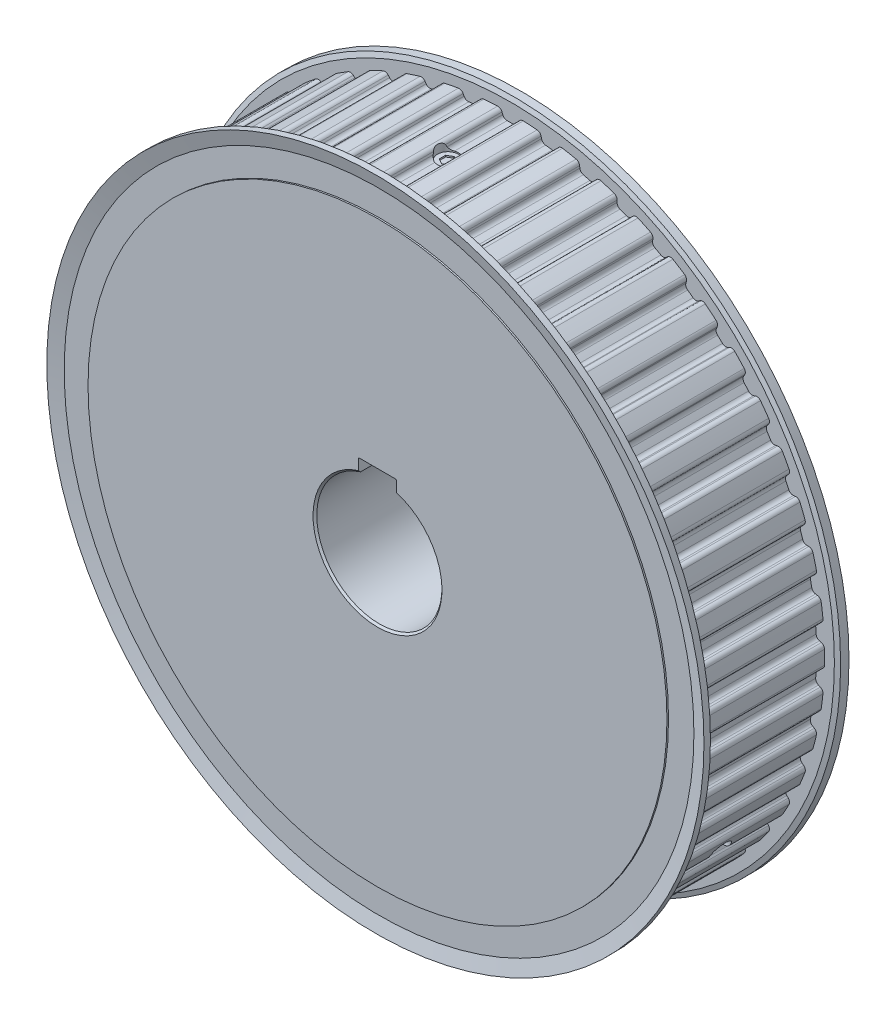
from build123d import *

# Parameters (mm, degrees)
CUT_EXTRUDE_1_DEPTH      = 20
CUT_EXTRUDE_1_DEPTH_BACK = 20
SKETCH_4_R               = 200.76
CUT_EXTRUDE_2_DEPTH      = 22.5
CUT_EXTRUDE_2_DEPTH_BACK = 22.5
SKETCH_8_W               = 3.3235
SKETCH_8_H               = 81.38
CUT_EXTRUDE_3_DEPTH      = 0.5
CUT_EXTRUDE_4_DEPTH      = 0.5


with BuildPart() as part:
    # 草图1 → 旋转1 (revolve)
    with BuildSketch(Plane(origin=(0, 0, 0), x_dir=(0, 0, -1), z_dir=(1, 0, 0)), mode=Mode.PRIVATE) as revolve_1_sk:
        Polygon((0, 0), (0, 92.5), (2.5, 92.5), (2.5, 102.38), (42.5, 102.38), (42.5, 92.5), (45, 92.5), (45, 0), align=None)
    revolve(revolve_1_sk.sketch.rotate(Axis((0, 0, -45), (0, 0, 1)), 270), axis=Axis((0, 0, -45), (0, 0, 1)))

    # 草图2 → 切除-旋转1 (revolve, cut)
    with BuildSketch(Plane(origin=(0, 0, 0), x_dir=(0, 0, -1), z_dir=(1, 0, 0)), mode=Mode.PRIVATE) as cut_revolve_1_sk:
        Polygon((0, 0), (0, 20.6), (0.6, 20), (44.4, 20), (45, 20.6), (45, 0), align=None)
    revolve(cut_revolve_1_sk.sketch.rotate(Axis((0, 0, -45), (0, 0, 1)), 270), axis=Axis((0, 0, -45), (0, 0, 1)), mode=Mode.SUBTRACT)

    # 草图3 → 旋转2 (revolve)
    with BuildSketch(Plane(origin=(0, 0, 0), x_dir=(0, 0, -1), z_dir=(1, 0, 0)), mode=Mode.PRIVATE) as revolve_2_sk:
        Polygon((42.5, 103.5), (42.5, 92.5), (44.5, 92.5), (44.5, 105), (43, 105), align=None)
    revolve(revolve_2_sk.sketch.rotate(Axis((0, 0, -50), (0, 0, 1)), 270), axis=Axis((0, 0, -50), (0, 0, 1)))

    # 草图4 → 切除-拉伸1 (cut, two sides: drawn at the far end of the back side and taken through both)
    with BuildSketch(Plane.XY.offset(-22.5).offset(-CUT_EXTRUDE_1_DEPTH_BACK)):
        Circle(SKETCH_4_R)
        with BuildLine():
            Line((-99.336884651, -3.543386548), (-98.711914642, -3.727325224))
            ThreePointArc((-98.711914642, -3.727325224), (-97.97307181, -4.226775349), (-97.658926902, -5.061432245))
            ThreePointArc((-97.658926902, -5.061432245), (-97.597033773, -6.140284905), (-97.523222764, -7.218387755))
            ThreePointArc((-97.523222764, -7.218387755), (-97.730280298, -8.085835929), (-98.400699434, -8.673949302))
            Line((-98.400699434, -8.673949302), (-98.997687739, -8.934767079))
            ThreePointArc((-98.997687739, -8.934767079), (-99.656069764, -9.521039759), (-99.841575427, -10.382880925))
            ThreePointArc((-99.841575427, -10.382880925), (-99.588473718, -12.580949985), (-99.286986225, -14.772906499))
            ThreePointArc((-99.286986225, -14.772906499), (-98.892977381, -15.561537958), (-98.109479551, -15.965658852))
            Line((-98.109479551, -15.965658852), (-97.466383988, -16.069817605))
            ThreePointArc((-97.466383988, -16.069817605), (-96.670769454, -16.472727855), (-96.254491424, -17.261430435))
            ThreePointArc((-96.254491424, -17.261430435), (-96.057870249, -18.324018753), (-95.849519145, -19.384369468))
            ThreePointArc((-95.849519145, -19.384369468), (-95.946223884, -20.270928745), (-96.537646414, -20.938430466))
            Line((-96.537646414, -20.938430466), (-97.097238152, -21.272014092))
            ThreePointArc((-97.097238152, -21.272014092), (-97.676949188, -21.936180984), (-97.752974743, -22.8144763))
            ThreePointArc((-97.752974743, -22.8144763), (-97.226377714, -24.963490874), (-96.652542542, -27.100376754))
            ThreePointArc((-96.652542542, -27.100376754), (-96.162798845, -27.833407215), (-95.334829351, -28.136143178))
            Line((-95.334829351, -28.136143178), (-94.683750235, -28.158879362))
            ThreePointArc((-94.683750235, -28.158879362), (-93.843911315, -28.458895602), (-93.332065117, -29.189205555))
            ThreePointArc((-93.332065117, -29.189205555), (-93.003816729, -30.21877188), (-92.664211352, -31.244648095))
            ThreePointArc((-92.664211352, -31.244648095), (-92.649038204, -32.136336905), (-93.152137042, -32.872700074))
            Line((-93.152137042, -32.872700074), (-93.665507117, -33.273788735))
            ThreePointArc((-93.665507117, -33.273788735), (-94.157404774, -34.005375532), (-94.122751253, -34.886273755))
            ThreePointArc((-94.122751253, -34.886273755), (-93.330963653, -36.952342598), (-92.493830526, -39.000457877))
            ThreePointArc((-92.493830526, -39.000457877), (-91.916075526, -39.666327014), (-91.056691942, -39.86290372))
            Line((-91.056691942, -39.86290372), (-90.40789718, -39.803858771))
            ThreePointArc((-90.40789718, -39.803858771), (-89.537078635, -39.996249566), (-88.937736389, -40.656649468))
            ThreePointArc((-88.937736389, -40.656649468), (-88.483037461, -41.636956922), (-88.01753359, -42.612179957))
            ThreePointArc((-88.01753359, -42.612179957), (-87.890721846, -43.494935834), (-88.297562822, -44.288547564))
            Line((-88.297562822, -44.288547564), (-88.756615082, -44.750815853))
            ThreePointArc((-88.756615082, -44.750815853), (-89.15294184, -45.538284993), (-89.00815575, -46.407893833))
            ThreePointArc((-89.00815575, -46.407893833), (-87.963664543, -48.358433806), (-86.876435549, -50.285478483))
            ThreePointArc((-86.876435549, -50.285478483), (-86.219780788, -50.87368514), (-85.342536106, -50.961002456))
            Line((-85.342536106, -50.961002456), (-84.706257579, -50.821107549))
            ThreePointArc((-84.706257579, -50.821107549), (-83.818192738, -50.902838781), (-83.14080643, -51.48291373))
            ThreePointArc((-83.14080643, -51.48291373), (-82.566827835, -52.398502281), (-81.982766745, -53.307692286))
            ThreePointArc((-81.982766745, -53.307692286), (-81.7463163, -54.167593643), (-82.05048329, -55.005938202))
            Line((-82.05048329, -55.005938202), (-82.447978207, -55.522095872))
            ThreePointArc((-82.447978207, -55.522095872), (-82.742483756, -56.353028497), (-82.489848459, -57.197633703))
            ThreePointArc((-82.489848459, -57.197633703), (-81.209125895, -59.001883625), (-79.888947287, -60.777467053))
            ThreePointArc((-79.888947287, -60.777467053), (-79.163748602, -61.27873486), (-78.282477495, -61.255415741))
            Line((-78.282477495, -61.255415741), (-77.668749695, -61.036877102))
            ThreePointArc((-77.668749695, -61.036877102), (-76.777443871, -61.00665982), (-76.032696287, -61.49726169))
            ThreePointArc((-76.032696287, -61.49726169), (-75.348490011, -62.333691958), (-74.655082694, -63.162510463))
            ThreePointArc((-74.655082694, -63.162510463), (-74.312722514, -63.985996142), (-74.509418622, -64.855852336))
            Line((-74.509418622, -64.855852336), (-74.839087463, -65.417759272))
            ThreePointArc((-74.839087463, -65.417759272), (-75.027127275, -66.279051078), (-74.670626981, -67.08533272))
            ThreePointArc((-74.670626981, -67.08533272), (-73.173870821, -68.714838493), (-71.641562602, -70.310958662))
            ThreePointArc((-71.641562602, -70.310958662), (-70.859256811, -70.717382326), (-69.98785745, -70.583794528))
            Line((-69.98785745, -70.583794528), (-69.406359232, -70.290058641))
            ThreePointArc((-69.406359232, -70.290058641), (-68.525868849, -70.148369391), (-67.725505104, -70.541761095))
            ThreePointArc((-67.725505104, -70.541761095), (-66.941861489, -71.285842076), (-66.150043392, -72.021218118))
            ThreePointArc((-66.150043392, -72.021218118), (-65.707172702, -72.795301258), (-65.793295912, -73.682950936))
            Line((-65.793295912, -73.682950936), (-66.049939602, -74.281745529))
            ThreePointArc((-66.049939602, -74.281745529), (-66.128548178, -75.15981343), (-65.67380511, -75.915055966))
            ThreePointArc((-65.67380511, -75.915055966), (-63.984620091, -77.34411931), (-62.264347679, -78.73560445))
            ThreePointArc((-62.264347679, -78.73560445), (-61.43727221, -79.040774429), (-60.589487084, -78.79902471))
            Line((-60.589487084, -78.79902471), (-60.049389021, -78.434723967))
            ThreePointArc((-60.049389021, -78.434723967), (-59.193599941, -78.183797272), (-58.350242248, -78.473774788))
            ThreePointArc((-58.350242248, -78.473774788), (-57.479519822, -79.11377188), (-56.60177839, -79.74410814))
            ThreePointArc((-56.60177839, -79.74410814), (-56.065381524, -80.456580988), (-56.039573623, -81.348025383))
            Line((-56.039573623, -81.348025383), (-56.219144739, -81.974264286))
            ThreePointArc((-56.219144739, -81.974264286), (-56.187082372, -82.855260626), (-55.6412681, -83.54755343))
            ThreePointArc((-55.6412681, -83.54755343), (-53.78629368, -84.753637162), (-51.905186797, -85.918542722))
            ThreePointArc((-51.905186797, -85.918542722), (-51.046385126, -86.117646301), (-50.235584313, -85.7715472))
            Line((-50.235584313, -85.7715472), (-49.745404075, -85.34242684))
            ThreePointArc((-49.745404075, -85.34242684), (-48.9278126, -84.986219965), (-48.054761216, -85.168210176))
            ThreePointArc((-48.054761216, -85.168210176), (-47.11069179, -85.694030241), (-46.160869531, -86.20938594))
            ThreePointArc((-46.160869531, -86.20938594), (-45.539405788, -86.849012373), (-45.402073781, -87.730192875))
            Line((-45.402073781, -87.730192875), (-45.501740378, -88.373999926))
            ThreePointArc((-45.501740378, -88.373999926), (-45.359512714, -89.244030866), (-44.731235054, -89.862456068))
            ThreePointArc((-44.731235054, -89.862456068), (-42.739725287, -90.826539527), (-40.727450114, -91.74649425))
            ThreePointArc((-40.727450114, -91.74649425), (-39.850466054, -91.836391448), (-39.089436367, -91.391401154))
            Line((-39.089436367, -91.391401154), (-38.656904389, -90.904228662))
            ThreePointArc((-38.656904389, -90.904228662), (-37.890404427, -90.448359201), (-37.001427892, -90.519492011))
            ThreePointArc((-37.001427892, -90.519492011), (-35.998900007, -90.922842555), (-34.991976183, -91.315090225))
            ThreePointArc((-34.991976183, -91.315090225), (-34.295246419, -91.871782952), (-34.048556114, -92.728802818))
            Line((-34.048556114, -92.728802818), (-34.066746391, -93.380024795))
            ThreePointArc((-34.066746391, -93.380024795), (-33.816596443, -94.225369428), (-33.115763711, -94.760174092))
            ThreePointArc((-33.115763711, -94.760174092), (-31.019125895, -95.467053106), (-28.907417212, -96.127548757))
            ThreePointArc((-28.907417212, -96.127548757), (-28.026081328, -96.106821841), (-27.326824659, -95.569958116))
            Line((-27.326824659, -95.569958116), (-26.958762229, -95.032416494))
            ThreePointArc((-26.958762229, -95.032416494), (-26.255441942, -94.484073781), (-25.364559947, -94.443227384))
            ThreePointArc((-25.364559947, -94.443227384), (-24.319384066, -94.717747327), (-23.271238468, -94.980700988))
            ThreePointArc((-23.271238468, -94.980700988), (-22.510230527, -95.445680632), (-22.158072378, -96.265024147))
            Line((-22.158072378, -96.265024147), (-22.094499463, -96.91339089))
            ThreePointArc((-22.094499463, -96.91339089), (-21.740372245, -97.720717627), (-20.97803699, -98.163467563))
            ThreePointArc((-20.97803699, -98.163467563), (-18.809336358, -98.601994228), (-16.631497073, -98.992614397))
            ThreePointArc((-16.631497073, -98.992614397), (-15.759708557, -98.861590242), (-15.133252603, -98.241319749))
            Line((-15.133252603, -98.241319749), (-14.835464284, -97.661886348))
            ThreePointArc((-14.835464284, -97.661886348), (-14.206415453, -97.029718075), (-13.327677739, -96.877536643))
            ThreePointArc((-13.327677739, -96.877536643), (-12.25633691, -97.018896642), (-11.183499421, -97.148409358))
            ThreePointArc((-11.183499421, -97.148409358), (-10.370214852, -97.514342913), (-9.918142603, -98.28308854))
            Line((-9.918142603, -98.28308854), (-9.773809079, -98.918374918))
            ThreePointArc((-9.773809079, -98.918374918), (-9.32128939, -99.674951733), (-8.509474095, -100.018664511))
            ThreePointArc((-8.509474095, -100.018664511), (-6.30291235, -100.181923), (-4.09328829, -100.296507372))
            ThreePointArc((-4.09328829, -100.296507372), (-3.244795767, -100.057252307), (-2.701020112, -99.363357082))
            Line((-2.701020112, -99.363357082), (-2.478202205, -98.751169914))
            ThreePointArc((-2.478202205, -98.751169914), (-1.933345306, -98.045145753), (-1.080610092, -97.784029278))
            ThreePointArc((-1.080610092, -97.784029278), (0, -97.79), (1.080610092, -97.784029278))
            ThreePointArc((1.080610092, -97.784029278), (1.933345306, -98.045145753), (2.478202205, -98.751169914))
            Line((2.478202205, -98.751169914), (2.701020112, -99.363357082))
            ThreePointArc((2.701020112, -99.363357082), (3.244795767, -100.057252307), (4.09328829, -100.296507372))
            ThreePointArc((4.09328829, -100.296507372), (6.30291235, -100.181923), (8.509474095, -100.018664511))
            ThreePointArc((8.509474095, -100.018664511), (9.32128939, -99.674951733), (9.773809079, -98.918374918))
            Line((9.773809079, -98.918374918), (9.918142603, -98.28308854))
            ThreePointArc((9.918142603, -98.28308854), (10.370214852, -97.514342913), (11.183499421, -97.148409358))
            ThreePointArc((11.183499421, -97.148409358), (12.25633691, -97.018896642), (13.327677739, -96.877536643))
            ThreePointArc((13.327677739, -96.877536643), (14.206415453, -97.029718075), (14.835464284, -97.661886348))
            Line((14.835464284, -97.661886348), (15.133252603, -98.241319749))
            ThreePointArc((15.133252603, -98.241319749), (15.759708557, -98.861590242), (16.631497073, -98.992614397))
            ThreePointArc((16.631497073, -98.992614397), (18.809336358, -98.601994228), (20.97803699, -98.163467563))
            ThreePointArc((20.97803699, -98.163467563), (21.740372245, -97.720717627), (22.094499463, -96.91339089))
            Line((22.094499463, -96.91339089), (22.158072378, -96.265024147))
            ThreePointArc((22.158072378, -96.265024147), (22.510230527, -95.445680632), (23.271238468, -94.980700988))
            ThreePointArc((23.271238468, -94.980700988), (24.319384066, -94.717747327), (25.364559947, -94.443227384))
            ThreePointArc((25.364559947, -94.443227384), (26.255441942, -94.484073781), (26.958762229, -95.032416494))
            Line((26.958762229, -95.032416494), (27.326824659, -95.569958116))
            ThreePointArc((27.326824659, -95.569958116), (28.026081328, -96.106821841), (28.907417212, -96.127548757))
            ThreePointArc((28.907417212, -96.127548757), (31.019125895, -95.467053106), (33.115763711, -94.760174092))
            ThreePointArc((33.115763711, -94.760174092), (33.816596443, -94.225369428), (34.066746391, -93.380024795))
            Line((34.066746391, -93.380024795), (34.048556114, -92.728802818))
            ThreePointArc((34.048556114, -92.728802818), (34.295246419, -91.871782952), (34.991976183, -91.315090225))
            ThreePointArc((34.991976183, -91.315090225), (35.998900007, -90.922842555), (37.001427892, -90.519492011))
            ThreePointArc((37.001427892, -90.519492011), (37.890404427, -90.448359201), (38.656904389, -90.904228662))
            Line((38.656904389, -90.904228662), (39.089436367, -91.391401154))
            ThreePointArc((39.089436367, -91.391401154), (39.850466054, -91.836391448), (40.727450114, -91.74649425))
            ThreePointArc((40.727450114, -91.74649425), (42.739725287, -90.826539527), (44.731235054, -89.862456068))
            ThreePointArc((44.731235054, -89.862456068), (45.359512714, -89.244030866), (45.501740378, -88.373999926))
            Line((45.501740378, -88.373999926), (45.402073781, -87.730192875))
            ThreePointArc((45.402073781, -87.730192875), (45.539405788, -86.849012373), (46.160869531, -86.20938594))
            ThreePointArc((46.160869531, -86.20938594), (47.11069179, -85.694030241), (48.054761216, -85.168210176))
            ThreePointArc((48.054761216, -85.168210176), (48.9278126, -84.986219965), (49.745404075, -85.34242684))
            Line((49.745404075, -85.34242684), (50.235584313, -85.7715472))
            ThreePointArc((50.235584313, -85.7715472), (51.046385126, -86.117646301), (51.905186797, -85.918542722))
            ThreePointArc((51.905186797, -85.918542722), (53.78629368, -84.753637162), (55.6412681, -83.54755343))
            ThreePointArc((55.6412681, -83.54755343), (56.187082372, -82.855260626), (56.219144739, -81.974264286))
            Line((56.219144739, -81.974264286), (56.039573623, -81.348025383))
            ThreePointArc((56.039573623, -81.348025383), (56.065381524, -80.456580988), (56.60177839, -79.74410814))
            ThreePointArc((56.60177839, -79.74410814), (57.479519822, -79.11377188), (58.350242248, -78.473774788))
            ThreePointArc((58.350242248, -78.473774788), (59.193599941, -78.183797272), (60.049389021, -78.434723967))
            Line((60.049389021, -78.434723967), (60.589487084, -78.79902471))
            ThreePointArc((60.589487084, -78.79902471), (61.43727221, -79.040774429), (62.264347679, -78.73560445))
            ThreePointArc((62.264347679, -78.73560445), (63.984620091, -77.34411931), (65.67380511, -75.915055966))
            ThreePointArc((65.67380511, -75.915055966), (66.128548178, -75.15981343), (66.049939602, -74.281745529))
            Line((66.049939602, -74.281745529), (65.793295912, -73.682950936))
            ThreePointArc((65.793295912, -73.682950936), (65.707172702, -72.795301258), (66.150043392, -72.021218118))
            ThreePointArc((66.150043392, -72.021218118), (66.941861489, -71.285842076), (67.725505104, -70.541761095))
            ThreePointArc((67.725505104, -70.541761095), (68.525868849, -70.148369391), (69.406359232, -70.290058641))
            Line((69.406359232, -70.290058641), (69.98785745, -70.583794528))
            ThreePointArc((69.98785745, -70.583794528), (70.859256811, -70.717382326), (71.641562602, -70.310958662))
            ThreePointArc((71.641562602, -70.310958662), (73.173870821, -68.714838493), (74.670626981, -67.08533272))
            ThreePointArc((74.670626981, -67.08533272), (75.027127275, -66.279051078), (74.839087463, -65.417759272))
            Line((74.839087463, -65.417759272), (74.509418622, -64.855852336))
            ThreePointArc((74.509418622, -64.855852336), (74.312722514, -63.985996142), (74.655082694, -63.162510463))
            ThreePointArc((74.655082694, -63.162510463), (75.348490011, -62.333691958), (76.032696287, -61.49726169))
            ThreePointArc((76.032696287, -61.49726169), (76.777443871, -61.00665982), (77.668749695, -61.036877102))
            Line((77.668749695, -61.036877102), (78.282477495, -61.255415741))
            ThreePointArc((78.282477495, -61.255415741), (79.163748602, -61.27873486), (79.888947287, -60.777467053))
            ThreePointArc((79.888947287, -60.777467053), (81.209125895, -59.001883625), (82.489848459, -57.197633703))
            ThreePointArc((82.489848459, -57.197633703), (82.742483756, -56.353028497), (82.447978207, -55.522095872))
            Line((82.447978207, -55.522095872), (82.05048329, -55.005938202))
            ThreePointArc((82.05048329, -55.005938202), (81.7463163, -54.167593643), (81.982766745, -53.307692286))
            ThreePointArc((81.982766745, -53.307692286), (82.566827835, -52.398502281), (83.14080643, -51.48291373))
            ThreePointArc((83.14080643, -51.48291373), (83.818192738, -50.902838781), (84.706257579, -50.821107549))
            Line((84.706257579, -50.821107549), (85.342536106, -50.961002456))
            ThreePointArc((85.342536106, -50.961002456), (86.219780788, -50.87368514), (86.876435549, -50.285478483))
            ThreePointArc((86.876435549, -50.285478483), (87.963664543, -48.358433806), (89.00815575, -46.407893833))
            ThreePointArc((89.00815575, -46.407893833), (89.15294184, -45.538284993), (88.756615082, -44.750815853))
            Line((88.756615082, -44.750815853), (88.297562822, -44.288547564))
            ThreePointArc((88.297562822, -44.288547564), (87.890721846, -43.494935834), (88.01753359, -42.612179957))
            ThreePointArc((88.01753359, -42.612179957), (88.483037461, -41.636956922), (88.937736389, -40.656649468))
            ThreePointArc((88.937736389, -40.656649468), (89.537078635, -39.996249566), (90.40789718, -39.803858771))
            Line((90.40789718, -39.803858771), (91.056691942, -39.86290372))
            ThreePointArc((91.056691942, -39.86290372), (91.916075526, -39.666327014), (92.493830526, -39.000457877))
            ThreePointArc((92.493830526, -39.000457877), (93.330963653, -36.952342598), (94.122751253, -34.886273755))
            ThreePointArc((94.122751253, -34.886273755), (94.157404774, -34.005375532), (93.665507117, -33.273788735))
            Line((93.665507117, -33.273788735), (93.152137042, -32.872700074))
            ThreePointArc((93.152137042, -32.872700074), (92.649038204, -32.136336905), (92.664211352, -31.244648095))
            ThreePointArc((92.664211352, -31.244648095), (93.003816729, -30.21877188), (93.332065117, -29.189205555))
            ThreePointArc((93.332065117, -29.189205555), (93.843911315, -28.458895602), (94.683750235, -28.158879362))
            Line((94.683750235, -28.158879362), (95.334829351, -28.136143178))
            ThreePointArc((95.334829351, -28.136143178), (96.162798845, -27.833407215), (96.652542542, -27.100376754))
            ThreePointArc((96.652542542, -27.100376754), (97.226377714, -24.963490874), (97.752974743, -22.8144763))
            ThreePointArc((97.752974743, -22.8144763), (97.676949188, -21.936180984), (97.097238152, -21.272014092))
            Line((97.097238152, -21.272014092), (96.537646414, -20.938430466))
            ThreePointArc((96.537646414, -20.938430466), (95.946223884, -20.270928745), (95.849519145, -19.384369468))
            ThreePointArc((95.849519145, -19.384369468), (96.057870249, -18.324018753), (96.254491424, -17.261430435))
            ThreePointArc((96.254491424, -17.261430435), (96.670769454, -16.472727855), (97.466383988, -16.069817605))
            Line((97.466383988, -16.069817605), (98.109479551, -15.965658852))
            ThreePointArc((98.109479551, -15.965658852), (98.892977381, -15.561537958), (99.286986225, -14.772906499))
            ThreePointArc((99.286986225, -14.772906499), (99.588473718, -12.580949985), (99.841575427, -10.382880925))
            ThreePointArc((99.841575427, -10.382880925), (99.656069764, -9.521039759), (98.997687739, -8.934767079))
            Line((98.997687739, -8.934767079), (98.400699434, -8.673949302))
            ThreePointArc((98.400699434, -8.673949302), (97.730280298, -8.085835929), (97.523222764, -7.218387755))
            ThreePointArc((97.523222764, -7.218387755), (97.597033773, -6.140284905), (97.658926902, -5.061432245))
            ThreePointArc((97.658926902, -5.061432245), (97.97307181, -4.226775349), (98.711914642, -3.727325224))
            Line((98.711914642, -3.727325224), (99.336884651, -3.543386548))
            ThreePointArc((99.336884651, -3.543386548), (100.063554588, -3.044253951), (100.355614823, -2.212458685))
            ThreePointArc((100.355614823, -2.212458685), (100.38, 0), (100.355614823, 2.212458685))
            ThreePointArc((100.355614823, 2.212458685), (100.063554588, 3.044253951), (99.336884651, 3.543386548))
            Line((99.336884651, 3.543386548), (98.711914642, 3.727325224))
            ThreePointArc((98.711914642, 3.727325224), (97.97307181, 4.226775349), (97.658926902, 5.061432245))
            ThreePointArc((97.658926902, 5.061432245), (97.597033773, 6.140284905), (97.523222764, 7.218387755))
            ThreePointArc((97.523222764, 7.218387755), (97.730280298, 8.085835929), (98.400699434, 8.673949302))
            Line((98.400699434, 8.673949302), (98.997687739, 8.934767079))
            ThreePointArc((98.997687739, 8.934767079), (99.656069764, 9.521039759), (99.841575427, 10.382880925))
            ThreePointArc((99.841575427, 10.382880925), (99.588473718, 12.580949985), (99.286986225, 14.772906499))
            ThreePointArc((99.286986225, 14.772906499), (98.892977381, 15.561537958), (98.109479551, 15.965658852))
            Line((98.109479551, 15.965658852), (97.466383988, 16.069817605))
            ThreePointArc((97.466383988, 16.069817605), (96.670769454, 16.472727855), (96.254491424, 17.261430435))
            ThreePointArc((96.254491424, 17.261430435), (96.057870249, 18.324018753), (95.849519145, 19.384369468))
            ThreePointArc((95.849519145, 19.384369468), (95.946223884, 20.270928745), (96.537646414, 20.938430466))
            Line((96.537646414, 20.938430466), (97.097238152, 21.272014092))
            ThreePointArc((97.097238152, 21.272014092), (97.676949188, 21.936180984), (97.752974743, 22.8144763))
            ThreePointArc((97.752974743, 22.8144763), (97.226377714, 24.963490874), (96.652542542, 27.100376754))
            ThreePointArc((96.652542542, 27.100376754), (96.162798845, 27.833407215), (95.334829351, 28.136143178))
            Line((95.334829351, 28.136143178), (94.683750235, 28.158879362))
            ThreePointArc((94.683750235, 28.158879362), (93.843911315, 28.458895602), (93.332065117, 29.189205555))
            ThreePointArc((93.332065117, 29.189205555), (93.003816729, 30.21877188), (92.664211352, 31.244648095))
            ThreePointArc((92.664211352, 31.244648095), (92.649038204, 32.136336905), (93.152137042, 32.872700074))
            Line((93.152137042, 32.872700074), (93.665507117, 33.273788735))
            ThreePointArc((93.665507117, 33.273788735), (94.157404774, 34.005375532), (94.122751253, 34.886273755))
            ThreePointArc((94.122751253, 34.886273755), (93.330963653, 36.952342598), (92.493830526, 39.000457877))
            ThreePointArc((92.493830526, 39.000457877), (91.916075526, 39.666327014), (91.056691942, 39.86290372))
            Line((91.056691942, 39.86290372), (90.40789718, 39.803858771))
            ThreePointArc((90.40789718, 39.803858771), (89.537078635, 39.996249566), (88.937736389, 40.656649468))
            ThreePointArc((88.937736389, 40.656649468), (88.483037461, 41.636956922), (88.01753359, 42.612179957))
            ThreePointArc((88.01753359, 42.612179957), (87.890721846, 43.494935834), (88.297562822, 44.288547564))
            Line((88.297562822, 44.288547564), (88.756615082, 44.750815853))
            ThreePointArc((88.756615082, 44.750815853), (89.15294184, 45.538284993), (89.00815575, 46.407893833))
            ThreePointArc((89.00815575, 46.407893833), (87.963664543, 48.358433806), (86.876435549, 50.285478483))
            ThreePointArc((86.876435549, 50.285478483), (86.219780788, 50.87368514), (85.342536106, 50.961002456))
            Line((85.342536106, 50.961002456), (84.706257579, 50.821107549))
            ThreePointArc((84.706257579, 50.821107549), (83.818192738, 50.902838781), (83.14080643, 51.48291373))
            ThreePointArc((83.14080643, 51.48291373), (82.566827835, 52.398502281), (81.982766745, 53.307692286))
            ThreePointArc((81.982766745, 53.307692286), (81.7463163, 54.167593643), (82.05048329, 55.005938202))
            Line((82.05048329, 55.005938202), (82.447978207, 55.522095872))
            ThreePointArc((82.447978207, 55.522095872), (82.742483756, 56.353028497), (82.489848459, 57.197633703))
            ThreePointArc((82.489848459, 57.197633703), (81.209125895, 59.001883625), (79.888947287, 60.777467053))
            ThreePointArc((79.888947287, 60.777467053), (79.163748602, 61.27873486), (78.282477495, 61.255415741))
            Line((78.282477495, 61.255415741), (77.668749695, 61.036877102))
            ThreePointArc((77.668749695, 61.036877102), (76.777443871, 61.00665982), (76.032696287, 61.49726169))
            ThreePointArc((76.032696287, 61.49726169), (75.348490011, 62.333691958), (74.655082694, 63.162510463))
            ThreePointArc((74.655082694, 63.162510463), (74.312722514, 63.985996142), (74.509418622, 64.855852336))
            Line((74.509418622, 64.855852336), (74.839087463, 65.417759272))
            ThreePointArc((74.839087463, 65.417759272), (75.027127275, 66.279051078), (74.670626981, 67.08533272))
            ThreePointArc((74.670626981, 67.08533272), (73.173870821, 68.714838493), (71.641562602, 70.310958662))
            ThreePointArc((71.641562602, 70.310958662), (70.859256811, 70.717382326), (69.98785745, 70.583794528))
            Line((69.98785745, 70.583794528), (69.406359232, 70.290058641))
            ThreePointArc((69.406359232, 70.290058641), (68.525868849, 70.148369391), (67.725505104, 70.541761095))
            ThreePointArc((67.725505104, 70.541761095), (66.941861489, 71.285842076), (66.150043392, 72.021218118))
            ThreePointArc((66.150043392, 72.021218118), (65.707172702, 72.795301258), (65.793295912, 73.682950936))
            Line((65.793295912, 73.682950936), (66.049939602, 74.281745529))
            ThreePointArc((66.049939602, 74.281745529), (66.128548178, 75.15981343), (65.67380511, 75.915055966))
            ThreePointArc((65.67380511, 75.915055966), (63.984620091, 77.34411931), (62.264347679, 78.73560445))
            ThreePointArc((62.264347679, 78.73560445), (61.43727221, 79.040774429), (60.589487084, 78.79902471))
            Line((60.589487084, 78.79902471), (60.049389021, 78.434723967))
            ThreePointArc((60.049389021, 78.434723967), (59.193599941, 78.183797272), (58.350242248, 78.473774788))
            ThreePointArc((58.350242248, 78.473774788), (57.479519822, 79.11377188), (56.60177839, 79.74410814))
            ThreePointArc((56.60177839, 79.74410814), (56.065381524, 80.456580988), (56.039573623, 81.348025383))
            Line((56.039573623, 81.348025383), (56.219144739, 81.974264286))
            ThreePointArc((56.219144739, 81.974264286), (56.187082372, 82.855260626), (55.6412681, 83.54755343))
            ThreePointArc((55.6412681, 83.54755343), (53.78629368, 84.753637162), (51.905186797, 85.918542722))
            ThreePointArc((51.905186797, 85.918542722), (51.046385126, 86.117646301), (50.235584313, 85.7715472))
            Line((50.235584313, 85.7715472), (49.745404075, 85.34242684))
            ThreePointArc((49.745404075, 85.34242684), (48.9278126, 84.986219965), (48.054761216, 85.168210176))
            ThreePointArc((48.054761216, 85.168210176), (47.11069179, 85.694030241), (46.160869531, 86.20938594))
            ThreePointArc((46.160869531, 86.20938594), (45.539405788, 86.849012373), (45.402073781, 87.730192875))
            Line((45.402073781, 87.730192875), (45.501740378, 88.373999926))
            ThreePointArc((45.501740378, 88.373999926), (45.359512714, 89.244030866), (44.731235054, 89.862456068))
            ThreePointArc((44.731235054, 89.862456068), (42.739725287, 90.826539527), (40.727450114, 91.74649425))
            ThreePointArc((40.727450114, 91.74649425), (39.850466054, 91.836391448), (39.089436367, 91.391401154))
            Line((39.089436367, 91.391401154), (38.656904389, 90.904228662))
            ThreePointArc((38.656904389, 90.904228662), (37.890404427, 90.448359201), (37.001427892, 90.519492011))
            ThreePointArc((37.001427892, 90.519492011), (35.998900007, 90.922842555), (34.991976183, 91.315090225))
            ThreePointArc((34.991976183, 91.315090225), (34.295246419, 91.871782952), (34.048556114, 92.728802818))
            Line((34.048556114, 92.728802818), (34.066746391, 93.380024795))
            ThreePointArc((34.066746391, 93.380024795), (33.816596443, 94.225369428), (33.115763711, 94.760174092))
            ThreePointArc((33.115763711, 94.760174092), (31.019125895, 95.467053106), (28.907417212, 96.127548757))
            ThreePointArc((28.907417212, 96.127548757), (28.026081328, 96.106821841), (27.326824659, 95.569958116))
            Line((27.326824659, 95.569958116), (26.958762229, 95.032416494))
            ThreePointArc((26.958762229, 95.032416494), (26.255441942, 94.484073781), (25.364559947, 94.443227384))
            ThreePointArc((25.364559947, 94.443227384), (24.319384066, 94.717747327), (23.271238468, 94.980700988))
            ThreePointArc((23.271238468, 94.980700988), (22.510230527, 95.445680632), (22.158072378, 96.265024147))
            Line((22.158072378, 96.265024147), (22.094499463, 96.91339089))
            ThreePointArc((22.094499463, 96.91339089), (21.740372245, 97.720717627), (20.97803699, 98.163467563))
            ThreePointArc((20.97803699, 98.163467563), (18.809336358, 98.601994228), (16.631497073, 98.992614397))
            ThreePointArc((16.631497073, 98.992614397), (15.759708557, 98.861590242), (15.133252603, 98.241319749))
            Line((15.133252603, 98.241319749), (14.835464284, 97.661886348))
            ThreePointArc((14.835464284, 97.661886348), (14.206415453, 97.029718075), (13.327677739, 96.877536643))
            ThreePointArc((13.327677739, 96.877536643), (12.25633691, 97.018896642), (11.183499421, 97.148409358))
            ThreePointArc((11.183499421, 97.148409358), (10.370214852, 97.514342913), (9.918142603, 98.28308854))
            Line((9.918142603, 98.28308854), (9.773809079, 98.918374918))
            ThreePointArc((9.773809079, 98.918374918), (9.32128939, 99.674951733), (8.509474095, 100.018664511))
            ThreePointArc((8.509474095, 100.018664511), (6.30291235, 100.181923), (4.09328829, 100.296507372))
            ThreePointArc((4.09328829, 100.296507372), (3.244795767, 100.057252307), (2.701020112, 99.363357082))
            Line((2.701020112, 99.363357082), (2.478202205, 98.751169914))
            ThreePointArc((2.478202205, 98.751169914), (1.933345306, 98.045145753), (1.080610092, 97.784029278))
            ThreePointArc((1.080610092, 97.784029278), (0, 97.79), (-1.080610092, 97.784029278))
            ThreePointArc((-1.080610092, 97.784029278), (-1.933345306, 98.045145753), (-2.478202205, 98.751169914))
            Line((-2.478202205, 98.751169914), (-2.701020112, 99.363357082))
            ThreePointArc((-2.701020112, 99.363357082), (-3.244795767, 100.057252307), (-4.09328829, 100.296507372))
            ThreePointArc((-4.09328829, 100.296507372), (-6.30291235, 100.181923), (-8.509474095, 100.018664511))
            ThreePointArc((-8.509474095, 100.018664511), (-9.32128939, 99.674951733), (-9.773809079, 98.918374918))
            Line((-9.773809079, 98.918374918), (-9.918142603, 98.28308854))
            ThreePointArc((-9.918142603, 98.28308854), (-10.370214852, 97.514342913), (-11.183499421, 97.148409358))
            ThreePointArc((-11.183499421, 97.148409358), (-12.25633691, 97.018896642), (-13.327677739, 96.877536643))
            ThreePointArc((-13.327677739, 96.877536643), (-14.206415453, 97.029718075), (-14.835464284, 97.661886348))
            Line((-14.835464284, 97.661886348), (-15.133252603, 98.241319749))
            ThreePointArc((-15.133252603, 98.241319749), (-15.759708557, 98.861590242), (-16.631497073, 98.992614397))
            ThreePointArc((-16.631497073, 98.992614397), (-18.809336358, 98.601994228), (-20.97803699, 98.163467563))
            ThreePointArc((-20.97803699, 98.163467563), (-21.740372245, 97.720717627), (-22.094499463, 96.91339089))
            Line((-22.094499463, 96.91339089), (-22.158072378, 96.265024147))
            ThreePointArc((-22.158072378, 96.265024147), (-22.510230527, 95.445680632), (-23.271238468, 94.980700988))
            ThreePointArc((-23.271238468, 94.980700988), (-24.319384066, 94.717747327), (-25.364559947, 94.443227384))
            ThreePointArc((-25.364559947, 94.443227384), (-26.255441942, 94.484073781), (-26.958762229, 95.032416494))
            Line((-26.958762229, 95.032416494), (-27.326824659, 95.569958116))
            ThreePointArc((-27.326824659, 95.569958116), (-28.026081328, 96.106821841), (-28.907417212, 96.127548757))
            ThreePointArc((-28.907417212, 96.127548757), (-31.019125895, 95.467053106), (-33.115763711, 94.760174092))
            ThreePointArc((-33.115763711, 94.760174092), (-33.816596443, 94.225369428), (-34.066746391, 93.380024795))
            Line((-34.066746391, 93.380024795), (-34.048556114, 92.728802818))
            ThreePointArc((-34.048556114, 92.728802818), (-34.295246419, 91.871782952), (-34.991976183, 91.315090225))
            ThreePointArc((-34.991976183, 91.315090225), (-35.998900007, 90.922842555), (-37.001427892, 90.519492011))
            ThreePointArc((-37.001427892, 90.519492011), (-37.890404427, 90.448359201), (-38.656904389, 90.904228662))
            Line((-38.656904389, 90.904228662), (-39.089436367, 91.391401154))
            ThreePointArc((-39.089436367, 91.391401154), (-39.850466054, 91.836391448), (-40.727450114, 91.74649425))
            ThreePointArc((-40.727450114, 91.74649425), (-42.739725287, 90.826539527), (-44.731235054, 89.862456068))
            ThreePointArc((-44.731235054, 89.862456068), (-45.359512714, 89.244030866), (-45.501740378, 88.373999926))
            Line((-45.501740378, 88.373999926), (-45.402073781, 87.730192875))
            ThreePointArc((-45.402073781, 87.730192875), (-45.539405788, 86.849012373), (-46.160869531, 86.20938594))
            ThreePointArc((-46.160869531, 86.20938594), (-47.11069179, 85.694030241), (-48.054761216, 85.168210176))
            ThreePointArc((-48.054761216, 85.168210176), (-48.9278126, 84.986219965), (-49.745404075, 85.34242684))
            Line((-49.745404075, 85.34242684), (-50.235584313, 85.7715472))
            ThreePointArc((-50.235584313, 85.7715472), (-51.046385126, 86.117646301), (-51.905186797, 85.918542722))
            ThreePointArc((-51.905186797, 85.918542722), (-53.78629368, 84.753637162), (-55.6412681, 83.54755343))
            ThreePointArc((-55.6412681, 83.54755343), (-56.187082372, 82.855260626), (-56.219144739, 81.974264286))
            Line((-56.219144739, 81.974264286), (-56.039573623, 81.348025383))
            ThreePointArc((-56.039573623, 81.348025383), (-56.065381524, 80.456580988), (-56.60177839, 79.74410814))
            ThreePointArc((-56.60177839, 79.74410814), (-57.479519822, 79.11377188), (-58.350242248, 78.473774788))
            ThreePointArc((-58.350242248, 78.473774788), (-59.193599941, 78.183797272), (-60.049389021, 78.434723967))
            Line((-60.049389021, 78.434723967), (-60.589487084, 78.79902471))
            ThreePointArc((-60.589487084, 78.79902471), (-61.43727221, 79.040774429), (-62.264347679, 78.73560445))
            ThreePointArc((-62.264347679, 78.73560445), (-63.984620091, 77.34411931), (-65.67380511, 75.915055966))
            ThreePointArc((-65.67380511, 75.915055966), (-66.128548178, 75.15981343), (-66.049939602, 74.281745529))
            Line((-66.049939602, 74.281745529), (-65.793295912, 73.682950936))
            ThreePointArc((-65.793295912, 73.682950936), (-65.707172702, 72.795301258), (-66.150043392, 72.021218118))
            ThreePointArc((-66.150043392, 72.021218118), (-66.941861489, 71.285842076), (-67.725505104, 70.541761095))
            ThreePointArc((-67.725505104, 70.541761095), (-68.525868849, 70.148369391), (-69.406359232, 70.290058641))
            Line((-69.406359232, 70.290058641), (-69.98785745, 70.583794528))
            ThreePointArc((-69.98785745, 70.583794528), (-70.859256811, 70.717382326), (-71.641562602, 70.310958662))
            ThreePointArc((-71.641562602, 70.310958662), (-73.173870821, 68.714838493), (-74.670626981, 67.08533272))
            ThreePointArc((-74.670626981, 67.08533272), (-75.027127275, 66.279051078), (-74.839087463, 65.417759272))
            Line((-74.839087463, 65.417759272), (-74.509418622, 64.855852336))
            ThreePointArc((-74.509418622, 64.855852336), (-74.312722514, 63.985996142), (-74.655082694, 63.162510463))
            ThreePointArc((-74.655082694, 63.162510463), (-75.348490011, 62.333691958), (-76.032696287, 61.49726169))
            ThreePointArc((-76.032696287, 61.49726169), (-76.777443871, 61.00665982), (-77.668749695, 61.036877102))
            Line((-77.668749695, 61.036877102), (-78.282477495, 61.255415741))
            ThreePointArc((-78.282477495, 61.255415741), (-79.163748602, 61.27873486), (-79.888947287, 60.777467053))
            ThreePointArc((-79.888947287, 60.777467053), (-81.209125895, 59.001883625), (-82.489848459, 57.197633703))
            ThreePointArc((-82.489848459, 57.197633703), (-82.742483756, 56.353028497), (-82.447978207, 55.522095872))
            Line((-82.447978207, 55.522095872), (-82.05048329, 55.005938202))
            ThreePointArc((-82.05048329, 55.005938202), (-81.7463163, 54.167593643), (-81.982766745, 53.307692286))
            ThreePointArc((-81.982766745, 53.307692286), (-82.566827835, 52.398502281), (-83.14080643, 51.48291373))
            ThreePointArc((-83.14080643, 51.48291373), (-83.818192738, 50.902838781), (-84.706257579, 50.821107549))
            Line((-84.706257579, 50.821107549), (-85.342536106, 50.961002456))
            ThreePointArc((-85.342536106, 50.961002456), (-86.219780788, 50.87368514), (-86.876435549, 50.285478483))
            ThreePointArc((-86.876435549, 50.285478483), (-87.963664543, 48.358433806), (-89.00815575, 46.407893833))
            ThreePointArc((-89.00815575, 46.407893833), (-89.15294184, 45.538284993), (-88.756615082, 44.750815853))
            Line((-88.756615082, 44.750815853), (-88.297562822, 44.288547564))
            ThreePointArc((-88.297562822, 44.288547564), (-87.890721846, 43.494935834), (-88.01753359, 42.612179957))
            ThreePointArc((-88.01753359, 42.612179957), (-88.483037461, 41.636956922), (-88.937736389, 40.656649468))
            ThreePointArc((-88.937736389, 40.656649468), (-89.537078635, 39.996249566), (-90.40789718, 39.803858771))
            Line((-90.40789718, 39.803858771), (-91.056691942, 39.86290372))
            ThreePointArc((-91.056691942, 39.86290372), (-91.916075526, 39.666327014), (-92.493830526, 39.000457877))
            ThreePointArc((-92.493830526, 39.000457877), (-93.330963653, 36.952342598), (-94.122751253, 34.886273755))
            ThreePointArc((-94.122751253, 34.886273755), (-94.157404774, 34.005375532), (-93.665507117, 33.273788735))
            Line((-93.665507117, 33.273788735), (-93.152137042, 32.872700074))
            ThreePointArc((-93.152137042, 32.872700074), (-92.649038204, 32.136336905), (-92.664211352, 31.244648095))
            ThreePointArc((-92.664211352, 31.244648095), (-93.003816729, 30.21877188), (-93.332065117, 29.189205555))
            ThreePointArc((-93.332065117, 29.189205555), (-93.843911315, 28.458895602), (-94.683750235, 28.158879362))
            Line((-94.683750235, 28.158879362), (-95.334829351, 28.136143178))
            ThreePointArc((-95.334829351, 28.136143178), (-96.162798845, 27.833407215), (-96.652542542, 27.100376754))
            ThreePointArc((-96.652542542, 27.100376754), (-97.226377714, 24.963490874), (-97.752974743, 22.8144763))
            ThreePointArc((-97.752974743, 22.8144763), (-97.676949188, 21.936180984), (-97.097238152, 21.272014092))
            Line((-97.097238152, 21.272014092), (-96.537646414, 20.938430466))
            ThreePointArc((-96.537646414, 20.938430466), (-95.946223884, 20.270928745), (-95.849519145, 19.384369468))
            ThreePointArc((-95.849519145, 19.384369468), (-96.057870249, 18.324018753), (-96.254491424, 17.261430435))
            ThreePointArc((-96.254491424, 17.261430435), (-96.670769454, 16.472727855), (-97.466383988, 16.069817605))
            Line((-97.466383988, 16.069817605), (-98.109479551, 15.965658852))
            ThreePointArc((-98.109479551, 15.965658852), (-98.892977381, 15.561537958), (-99.286986225, 14.772906499))
            ThreePointArc((-99.286986225, 14.772906499), (-99.588473718, 12.580949985), (-99.841575427, 10.382880925))
            ThreePointArc((-99.841575427, 10.382880925), (-99.656069764, 9.521039759), (-98.997687739, 8.934767079))
            Line((-98.997687739, 8.934767079), (-98.400699434, 8.673949302))
            ThreePointArc((-98.400699434, 8.673949302), (-97.730280298, 8.085835929), (-97.523222764, 7.218387755))
            ThreePointArc((-97.523222764, 7.218387755), (-97.597033773, 6.140284905), (-97.658926902, 5.061432245))
            ThreePointArc((-97.658926902, 5.061432245), (-97.97307181, 4.226775349), (-98.711914642, 3.727325224))
            Line((-98.711914642, 3.727325224), (-99.336884651, 3.543386548))
            ThreePointArc((-99.336884651, 3.543386548), (-100.063554588, 3.044253951), (-100.355614823, 2.212458685))
            ThreePointArc((-100.355614823, 2.212458685), (-100.38, 0), (-100.355614823, -2.212458685))
            ThreePointArc((-100.355614823, -2.212458685), (-100.063554588, -3.044253951), (-99.336884651, -3.543386548))
        make_face(mode=Mode.SUBTRACT)
    extrude(amount=CUT_EXTRUDE_1_DEPTH + CUT_EXTRUDE_1_DEPTH_BACK, mode=Mode.SUBTRACT)

    # 草图5 → 切除-旋转2 (revolve, cut)
    with BuildSketch(Plane.XY.offset(-22.5), mode=Mode.PRIVATE) as cut_revolve_2_sk:
        Polygon((86.940288183, -50.195003642), (85.278538063, -53.073239002), (14.801392407, -12.383236049), (16.463142528, -9.50500069), align=None)
    revolve(cut_revolve_2_sk.sketch.rotate(Axis((16.463142528, -9.50500069, -22.5), (0.866025382840487, -0.5000000362759868, 0)), 180), axis=Axis((16.463142528, -9.50500069, -22.5), (0.866025382840487, -0.5000000362759868, 0)), mode=Mode.SUBTRACT)

    # 草图6 → 旋转3 (revolve)
    with BuildSketch(Plane.XY.offset(-22.5), mode=Mode.PRIVATE) as revolve_3_sk:
        Polygon((84.333553821, -48.69), (82.333553821, -52.154101615), (16.186533479, -13.964101615), (18.186533479, -10.5), align=None)
    revolve(revolve_3_sk.sketch.rotate(Axis((18.186533479, -10.5, -22.5), (0.8660254037844387, -0.49999999999999983, 0)), 88.098400493), axis=Axis((18.186533479, -10.5, -22.5), (0.8660254037844387, -0.49999999999999983, 0)))

    # 草图7 → 切除-拉伸2 (cut, two sides: drawn at the far end of the back side and taken through both)
    with BuildSketch(Plane.XY.offset(-22.5).offset(-CUT_EXTRUDE_2_DEPTH_BACK)):
        with BuildLine():
            Line((-6, 23.1), (-6, 18.869022232))
            ThreePointArc((-6, 18.869022232), (0, 19.8), (6, 18.869022232))
            Line((6, 18.869022232), (6, 23.1))
            ThreePointArc((6, 23.1), (5.941421356, 23.241421356), (5.8, 23.3))
            Line((5.8, 23.3), (-5.8, 23.3))
            ThreePointArc((-5.8, 23.3), (-5.941421356, 23.241421356), (-6, 23.1))
        make_face()
    extrude(amount=CUT_EXTRUDE_2_DEPTH + CUT_EXTRUDE_2_DEPTH_BACK, mode=Mode.SUBTRACT)

    # 草图8 → 切除-旋转3 (revolve, cut)
    with BuildSketch(Plane.XY.offset(-22.5), mode=Mode.PRIVATE) as cut_revolve_3_sk:
        with Locations((1.66175, 59.7)):
            Rectangle(SKETCH_8_W, SKETCH_8_H)
    revolve(cut_revolve_3_sk.sketch.rotate(Axis((0, 19.01, -22.5), (0, 1, 0)), 270), axis=Axis((0, 19.01, -22.5), (0, 1, 0)), mode=Mode.SUBTRACT)

    # 草图9 → 旋转4 (revolve)
    with BuildSketch(Plane.XY.offset(-22.5), mode=Mode.PRIVATE) as revolve_4_sk:
        Polygon((0, 97.38), (3.8, 97.38), (4, 97.18), (4, 24.5), (3.8, 24.3), (0, 24.3), align=None)
    revolve(revolve_4_sk.sketch.rotate(Axis((0, 24.3, -22.5), (0, 1, 0)), 288.974190184), axis=Axis((0, 24.3, -22.5), (0, 1, 0)))

    # 草图10 → 切除-拉伸3 (cut)
    with BuildSketch(Plane(origin=(0, 97.38, 0), x_dir=(1, 0, 0), z_dir=(0, 1, 0))):
        Polygon((-1.75, 21.489637029), (0, 20.479274058), (1.75, 21.489637029), (1.75, 23.510362971), (0, 24.520725942), (-1.75, 23.510362971), align=None)
    extrude(amount=-CUT_EXTRUDE_3_DEPTH, mode=Mode.SUBTRACT)

    # 草图11 → 切除-拉伸4 (cut)
    with BuildSketch(Plane(origin=(84.333553821, -48.69, 0), x_dir=(0, 0, -1), z_dir=(0.8660254037844386, -0.4999999999999999, 0))):
        Polygon((21.489637029, 1.75), (20.479274058, 0), (21.489637029, -1.75), (23.510362971, -1.75), (24.520725942, 0), (23.510362971, 1.75), align=None)
    extrude(amount=-CUT_EXTRUDE_4_DEPTH, mode=Mode.SUBTRACT)

    # 草图12 → 旋转5 (revolve)
    with BuildSketch(Plane(origin=(0, 0, 0), x_dir=(0, 0, -1), z_dir=(1, 0, 0)), mode=Mode.PRIVATE) as revolve_5_sk:
        Polygon((-0.674503034, 105), (0.5, 100.616695005), (0.5, 92.5), (2.5, 92.5), (2.5, 100.88), (1.396049327, 105), align=None)
    revolve(revolve_5_sk.sketch.rotate(Axis((0, 0, -50), (0, 0, 1)), 270), axis=Axis((0, 0, -50), (0, 0, 1)))

    # 草图13 → 旋转6 (revolve)
    with BuildSketch(Plane(origin=(0, 0, 0), x_dir=(0, 0, -1), z_dir=(1, 0, 0)), mode=Mode.PRIVATE) as revolve_6_sk:
        Polygon((42.5, 100.88), (42.5, 92.5), (44.5, 92.5), (44.5, 100.616695005), (45.674503034, 105), (43.603950673, 105), align=None)
    revolve(revolve_6_sk.sketch.rotate(Axis((0, 0, -50), (0, 0, 1)), 270), axis=Axis((0, 0, -50), (0, 0, 1)))


solid = part.part
